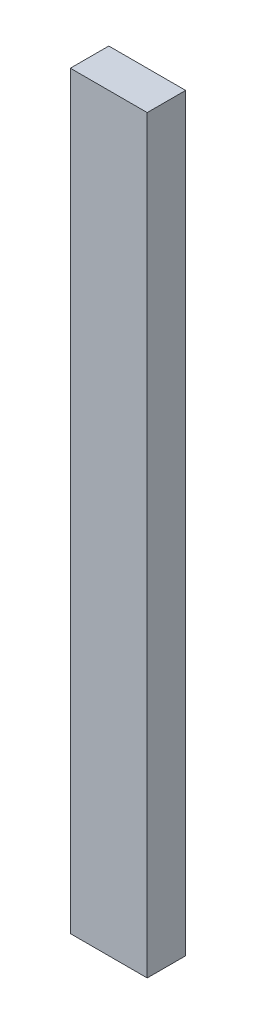
from build123d import *

# Parameters (mm, degrees)
SKETCH_1_W      = 20
SKETCH_1_H      = 195
EXTRUDE_1_DEPTH = 10


with BuildPart() as part:
    # 草图1 → 凸台-拉伸1 (new body)
    with BuildSketch(Plane.XY):
        Rectangle(SKETCH_1_W, SKETCH_1_H)
    extrude(amount=EXTRUDE_1_DEPTH)


solid = part.part
